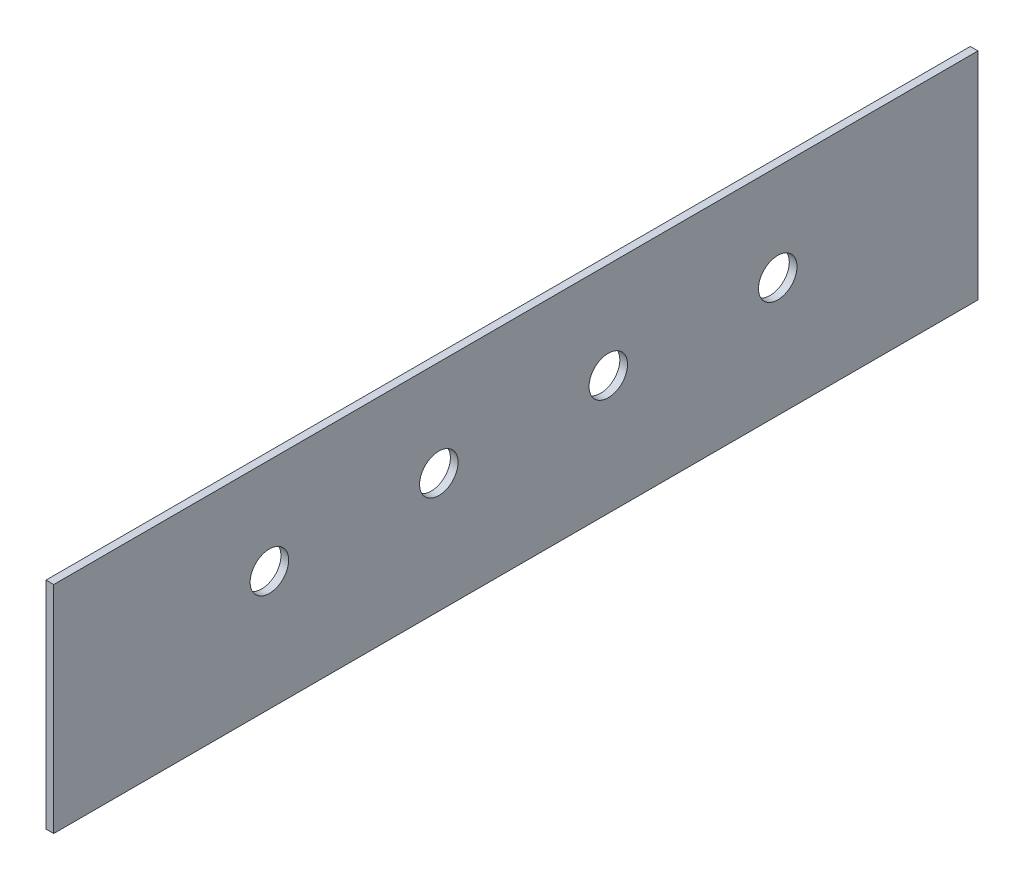
from build123d import *

# Parameters (mm, degrees)
SKETCH1_W           = 1200
SKETCH1_H           = 280
BOSS_EXTRUDE1_DEPTH = 10
SKETCH2_R           = 25
CUT_EXTRUDE1_DEPTH  = 10
LPATTERN1_COUNT     = 4
LPATTERN1_PITCH     = 220


with BuildPart() as part:
    # Sketch1 → Boss-Extrude1 (new body)
    with BuildSketch(Plane(origin=(0, 0, 0), x_dir=(0, 0, -1), z_dir=(1, 0, 0))):
        Rectangle(SKETCH1_W, SKETCH1_H)
    extrude(amount=BOSS_EXTRUDE1_DEPTH)

    # Sketch2 → Cut-Extrude1 (cut)
    with BuildSketch(Plane(origin=(10, 0, 0), x_dir=(0, 0, -1), z_dir=(1, 0, 0))):
        with Locations((-320, 15)):
            Circle(SKETCH2_R)
    cut_extrude1 = extrude(amount=-CUT_EXTRUDE1_DEPTH, mode=Mode.SUBTRACT)

    # LPattern1: Cut-Extrude1 ×4
    with Locations(*[(0, 0, -i * LPATTERN1_PITCH) for i in range(1, LPATTERN1_COUNT)]):
        add(cut_extrude1, mode=Mode.SUBTRACT)


solid = part.part
